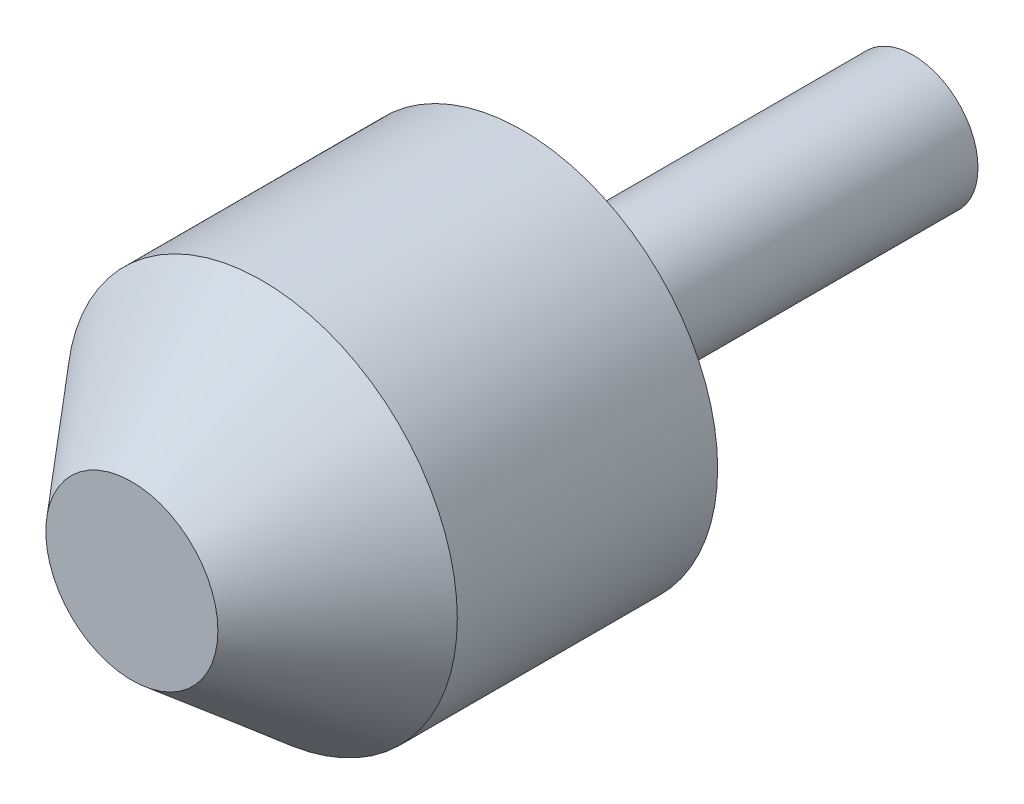
from build123d import *

# Parameters (mm, degrees)
SKETCH1_R           = 5
BOSS_EXTRUDE1_DEPTH = 30
SKETCH2_R           = 15
BOSS_EXTRUDE2_DEPTH = 30
CHAMFER1_SIZE       = 10
CHAMFER1_SIZE2      = 8.390996312


with BuildPart() as part:
    # Sketch1 → Boss-Extrude1 (new body)
    with BuildSketch(Plane.XY):
        Circle(SKETCH1_R)
    extrude(amount=BOSS_EXTRUDE1_DEPTH)

    # Sketch2 → Boss-Extrude2 (add)
    with BuildSketch(Plane.XY.offset(30)):
        Circle(SKETCH2_R)
    extrude(amount=BOSS_EXTRUDE2_DEPTH)

    # Chamfer1
    chamfer1_edges = [part.edges().sort_by_distance(p)[0] for p in [
        (-15, 0, 60),
    ]]
    chamfer1_side = [part.faces().sort_by_distance(p)[0] for p in [
        (-15, 0, 45),
    ]]
    chamfer(chamfer1_edges, length=CHAMFER1_SIZE, length2=CHAMFER1_SIZE2, reference=chamfer1_side[0])


solid = part.part
